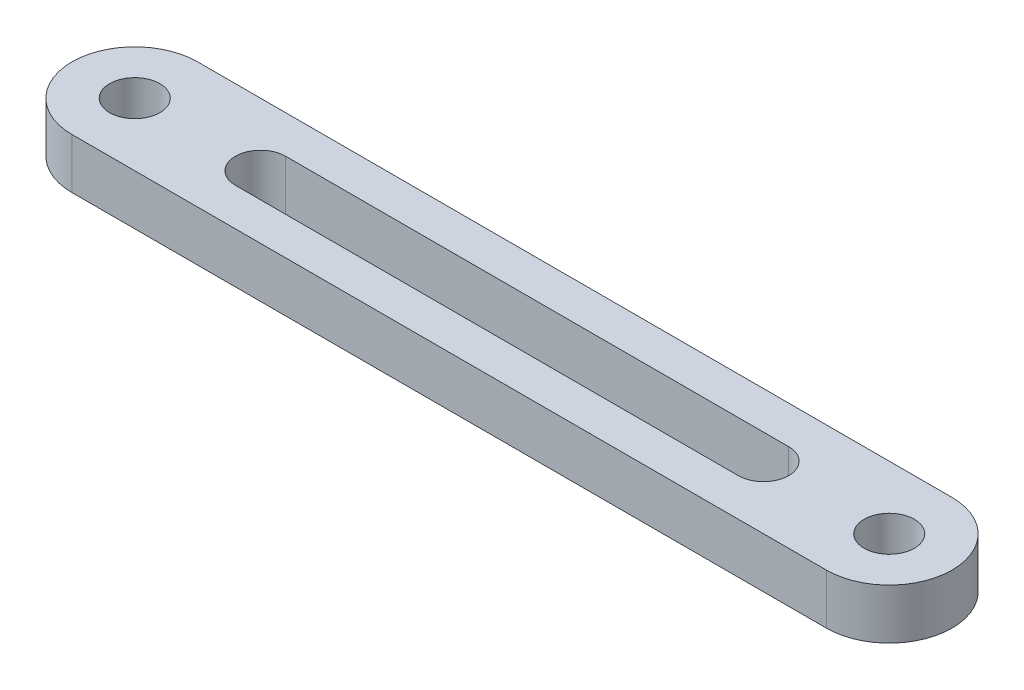
from build123d import *

# Parameters (mm, degrees)
SKETCH1_R           = 5
BOSS_EXTRUDE1_DEPTH = 5
CUT_EXTRUDE1_DEPTH  = 10


with BuildPart() as part:
    # Sketch1 → Boss-Extrude1 (new, symmetric)
    with BuildSketch(Plane(origin=(0, 0, 0), x_dir=(1, 0, 0), z_dir=(0, 1, 0))):
        with BuildLine():
            Line((0, 12.5), (150, 12.5))
            ThreePointArc((150, 12.5), (162.5, 0), (150, -12.5))
            Line((150, -12.5), (0, -12.5))
            ThreePointArc((0, -12.5), (-12.5, 0), (0, 12.5))
        make_face()
        with Locations(Location((0, 0, 0), (0, 0, 270))):
            Circle(SKETCH1_R, mode=Mode.SUBTRACT)
        with Locations(Location((150, 0, 0), (0, 0, 270))):
            Circle(SKETCH1_R, mode=Mode.SUBTRACT)
    extrude(amount=BOSS_EXTRUDE1_DEPTH, both=True)

    # Sketch2 → Cut-Extrude1 (cut)
    with BuildSketch(Plane(origin=(0, 5, 0), x_dir=(1, 0, 0), z_dir=(0, 1, 0))):
        with BuildLine():
            Line((25, 5), (125, 5))
            ThreePointArc((125, 5), (130, 0), (125, -5))
            Line((125, -5), (25, -5))
            ThreePointArc((25, -5), (20, 0), (25, 5))
        make_face()
    extrude(amount=-CUT_EXTRUDE1_DEPTH, mode=Mode.SUBTRACT)


solid = part.part
